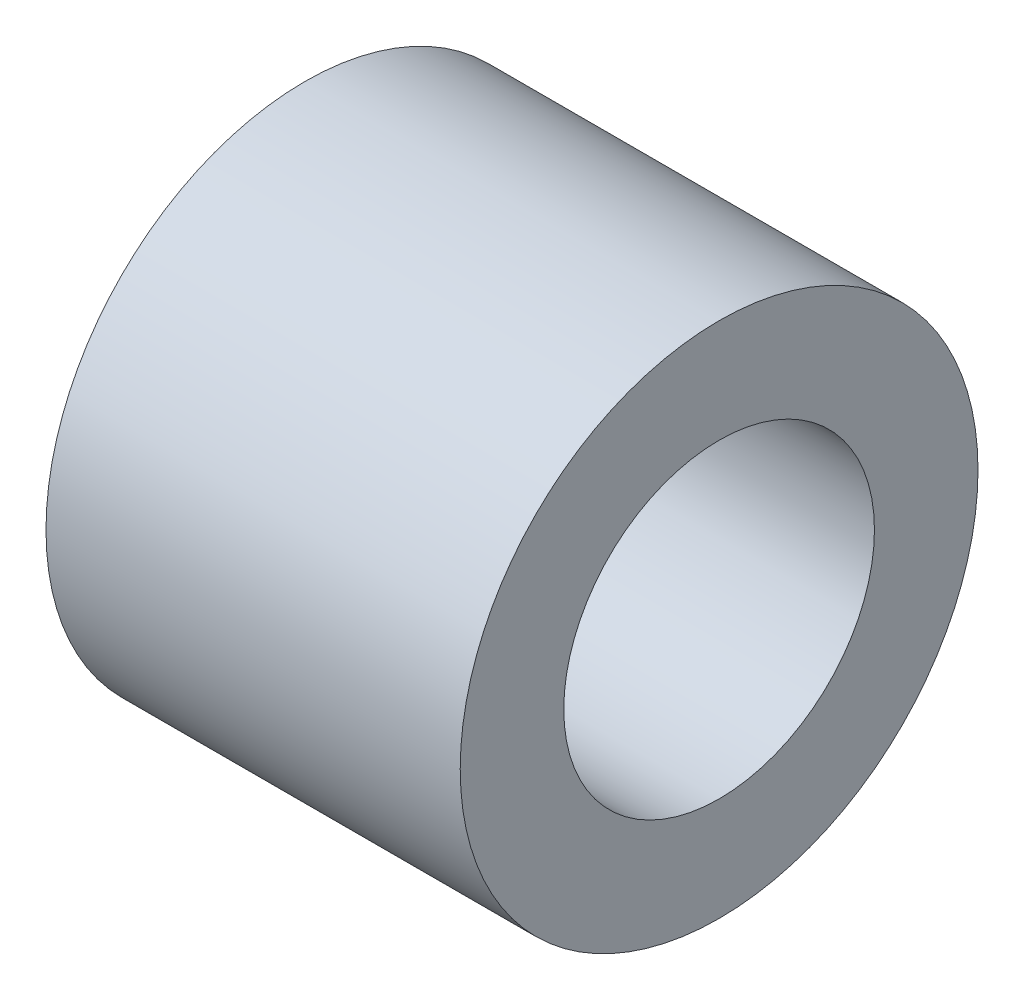
SolidWorks part; units mm, degrees
material "PU"
ref_plane "前基準面" through (0, 0, 0) normal (0, 0, 1) x (1, 0, 0)
ref_plane "上基準面" through (0, 0, 0) normal (0, 1, 0) x (1, 0, 0)
ref_plane "右基準面" through (0, 0, 0) normal (1, 0, 0) x (0, 0, -1)
sketch "草图1" plane through (0, 0, 0) normal (1, 0, 0) x (0, 0, -1)
  circle A0 centre (0, 0) radius 12.5
  dimension "D1" = 25
extrude "凸台-拉伸1" add sketch "草图1" along normal blind 20
hole_wizard "打孔尺寸(%根据)内六角圆柱头螺钉的类型1" positions "草图2" profile "草图3" counterbore size "M8" standard "GB" end condition through all
sketch "草图2" plane through (20, 0, 0) normal (1, 0, 0) x (0, 0, -1)
  point P0 (0, 0)
sketch "草图3" plane through (20, 0, 0) normal (0, 1, 0) x (0, 0, -1)
  line L0 (0, 0) -> (0, 20)
  line L1 (0, 20) -> (4.5, 20)
  line L3 (4.5, 20) -> (4.5, 12)
  line L4 (4.5, 12) -> (7.5, 12)
  line L5 (7.5, 12) -> (7.5, 0)
  line L7 (7.5, 0) -> (0, 0)
  line L11 (0, -6.35) -> (0, 107.95) construction
  dimension "通孔孔直径" = 9
  dimension "通孔孔深度" = 20
  dimension "柱形沉头孔直径" = 15
  dimension "柱形沉头孔深度" = 12
